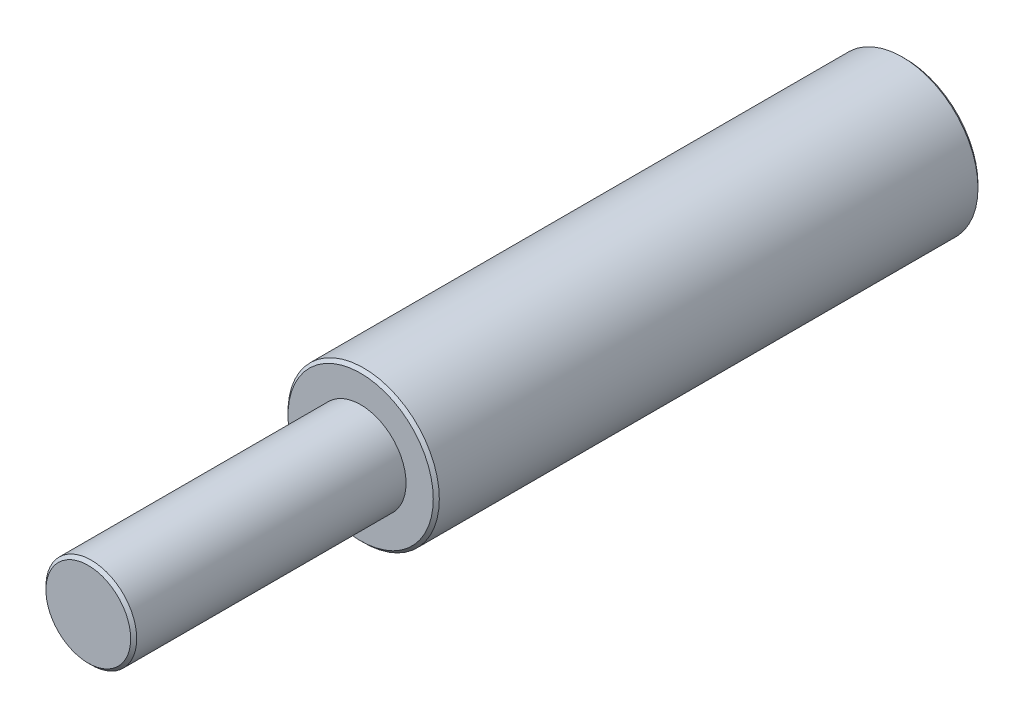
SolidWorks part; units mm, degrees
ref_plane "Front Plane" through (0, 0, 0) normal (0, 0, 1) x (1, 0, 0)
ref_plane "Top Plane" through (0, 0, 0) normal (0, 1, 0) x (1, 0, 0)
ref_plane "Right Plane" through (0, 0, 0) normal (1, 0, 0) x (0, 0, -1)
sketch "Sketch1" plane through (0, 0, 0) normal (0, 0, 1) x (1, 0, 0)
  circle A0 centre (0, 0) radius 25
  dimension "D1" = 50
extrude "Boss-Extrude1" add sketch "Sketch1" along normal blind 180
sketch "Sketch2" plane through (0, 0, 180) normal (0, 0, 1) x (1, 0, 0)
  circle A0 centre (0, 0) radius 15
  dimension "D1" = 30
extrude "Boss-Extrude2" add sketch "Sketch2" along normal blind 90
sketch "Sketch3" plane through (0, 0, 0) normal (0, 1, 0) x (1, 0, 0)
  line L0 (0, -84.2299) -> (0, -134.2299) construction
  line L1 (6, -84.2299) -> (6, -134.2299)
  line L2 (-6, -84.2299) -> (-6, -134.2299)
  arc A0 (6, -84.2299) -> (-6, -84.2299) centre (0, -84.2299) ccw
  arc A1 (-6, -134.2299) -> (6, -134.2299) centre (0, -134.2299) ccw
  point P3 (0, -109.2299)
  dimension "D1" = 12
  dimension "D2" = 50
extrude "Cut-Extrude1" cut sketch "Sketch3" against normal blind 120 from offset 20 offset against normal yes
chamfer "Chamfer1" distance 1 angle 45 3 edges at (25, 0, 180) (15, 0, 270) (25, 0, 0)
sketch "Sketch4" plane through (0, 0, 0) normal (1, 0, 0) x (0, 0, -1)
  line L0 (-270, 14) -> (-270, -14) construction
  circle A0 centre (-211, 0) radius 2.5
  dimension "D1" = 5
  dimension "D2" = 59
extrude "Cut-Extrude2" cut sketch "Sketch4" against normal blind 10 from offset 10
